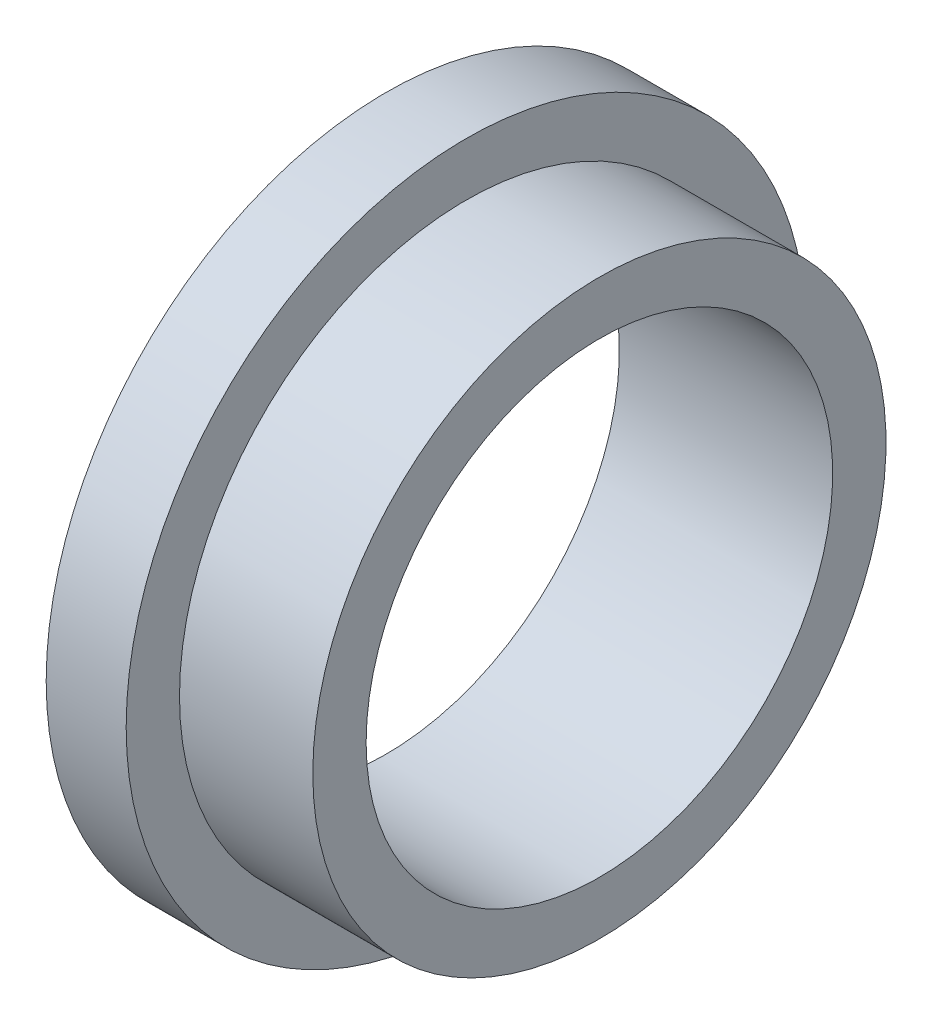
from build123d import *


with BuildPart() as part:
    # Sketch1 → Revolve1 (revolve)
    with BuildSketch(Plane.XY, mode=Mode.PRIVATE) as revolve1_sk:
        Polygon((-17.211842105, 17.5), (-5.342684211, 17.5), (-5.342684211, 21.5), (-15.342684211, 21.5), (-15.342684211, 25.5), (-21.342684211, 25.5), (-21.342684211, 17.5), align=None)
    revolve(revolve1_sk.sketch.rotate(Axis((0, 0, 0), (1, 0, 0)), 90), axis=Axis((0, 0, 0), (1, 0, 0)))


solid = part.part
